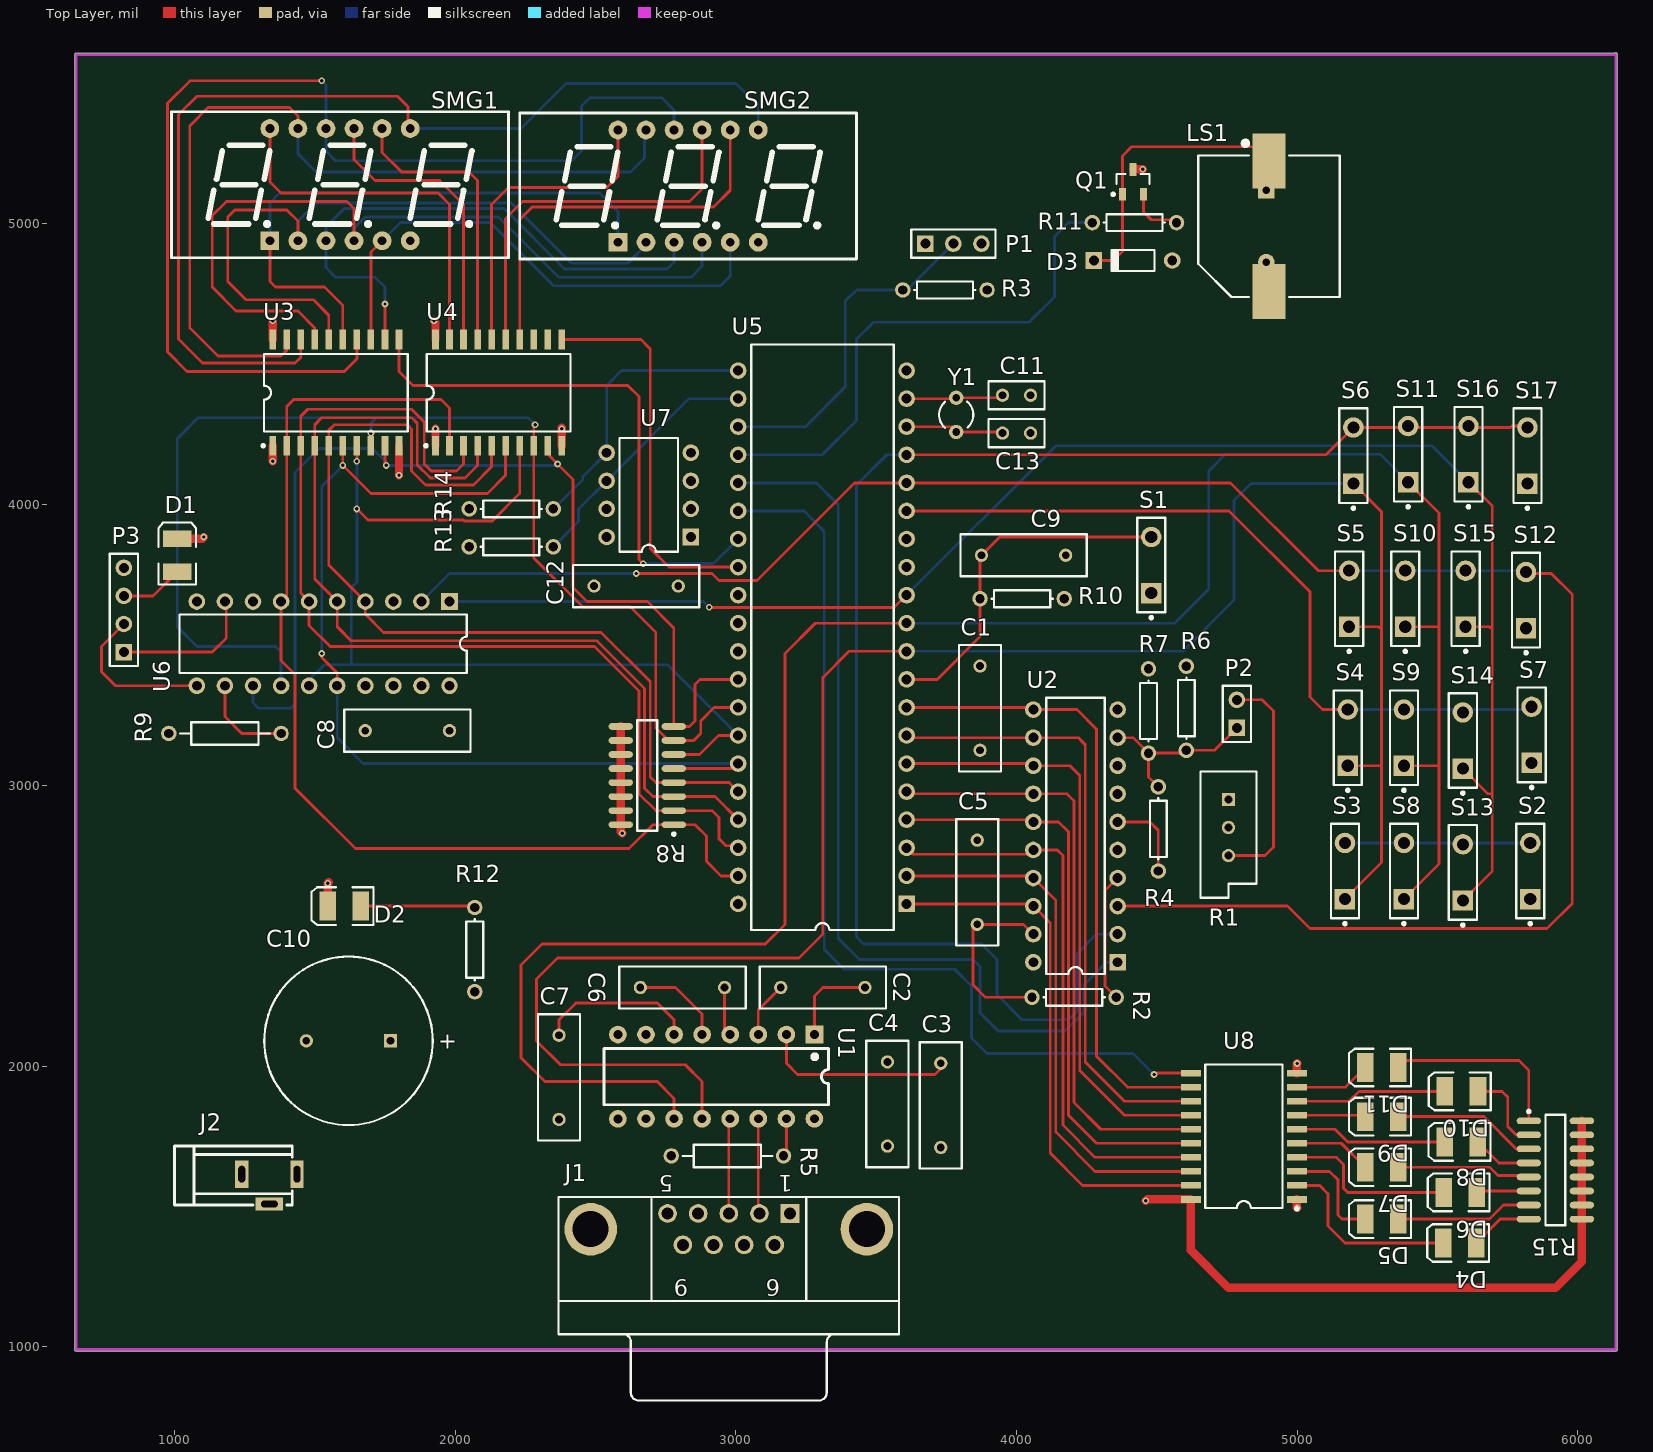
[diagram p0: Top Layer view]
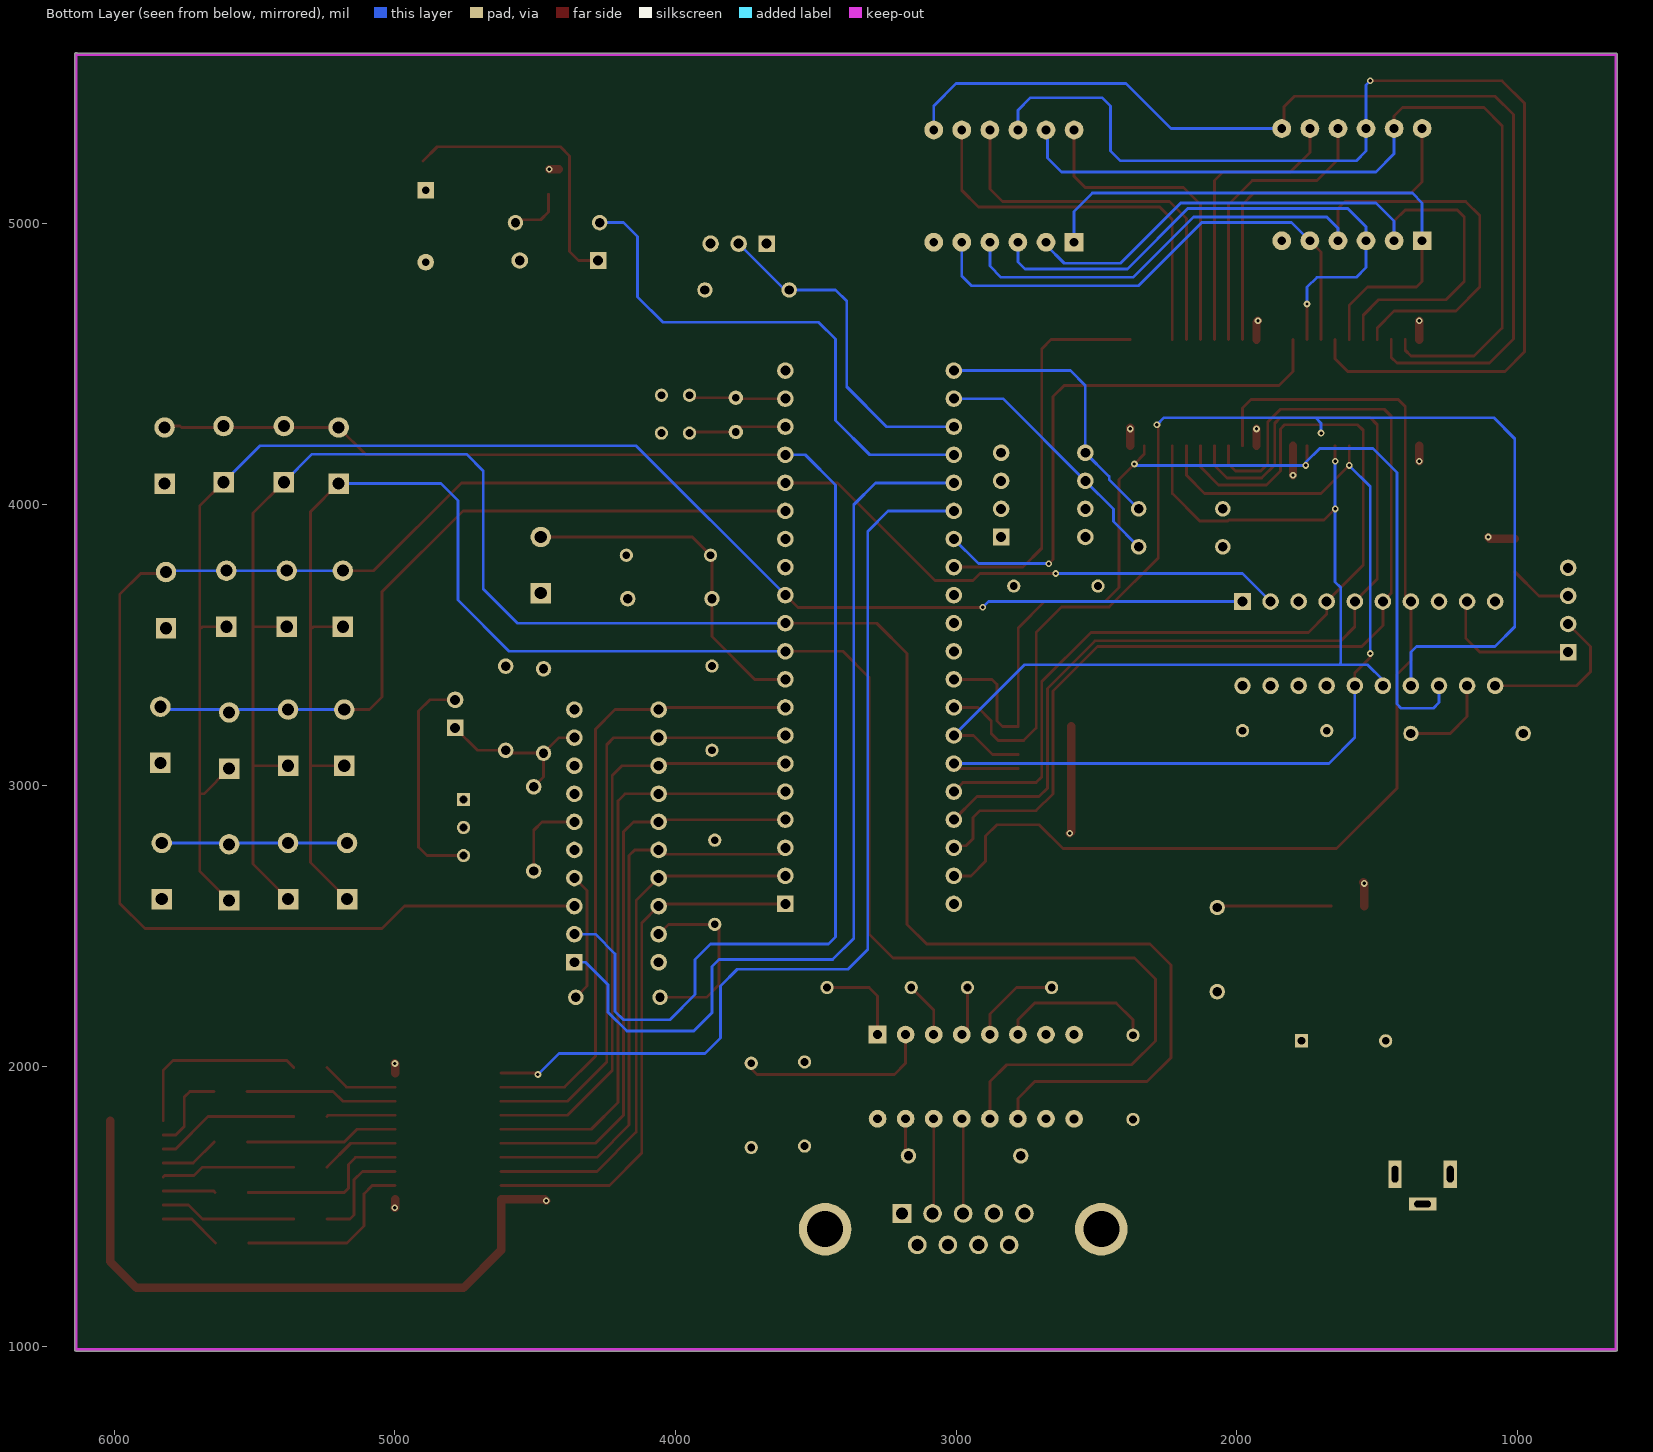
[diagram p1: Bottom Layer view, seen from below]
# Altium PCB MISC82251.PcbDoc (part 1 of 2)
Units mil, origin at the board's own origin, x right, y up, seen from the top; angles counter-clockwise.
Board outline 5495.03 x 4625.02 mil, 4 copper layers (Top Layer, VCC, GND, Bottom Layer), stack 30.634 mil thick; 74 components, 91 nets, 361 pads, 27 vias.

## Layer stack, top to bottom
Top Solder: solder mask 0.4, Solder Resist, Dk 3.5
Top Layer: signal copper 1.4
Dielectric 1: core 10, FR-4, Dk 4.2
VCC: signal copper 1.417
Dielectric 3: prepreg 5, Dk 4.2
GND: plane copper 1.417, net GND
Dielectric 2: core 10, Dk 4.2
Bottom Layer: signal copper 1.4
Bottom Solder: solder mask 0.4, Solder Resist, Dk 3.5

## Board outline
650,984.99 cw(c650,990) 644.99,990 644.99,5602.93 cw(c650,5602.93) 650,5607.94 6130,5607.94 ccw(c6130,5610) 6131.45,5608.55 cw(c6135,5605) 6140.02,5605 6140.02,990 cw(c6135,990) 6135,984.99

## Design rules (kind name [scope] priority, off if disabled: settings)
Clearance [All] p1: gap=10
HoleSize [All] p1: absolutevalues=TRUE maxlimit=10000 minlimit=1 maxpercent=80.000 minpercent=20.000
MinimumSolderMaskSliver [All] p1: minsoldermaskwidth=0
PlaneClearance [All] p1: clearance=20
PlaneConnect [All] p1: planeconnectstyle=Relief reliefexpansion=20 reliefentries=4 reliefconductorwidth=10 reliefairgap=10
PolygonConnect [All] p1: connectstyle=Relief reliefconductorwidth=10 reliefentries=4 polygonreliefangle="90 Angle" airgapwidth=10
RoutingVias [All] p1: holewidth=28 width=50 viastyle="Through Hole" minholewidth=28 minwidth=50 maxholewidth=28 maxwidth=50
SilkToSilkClearance [All] p1: silktosilkclearance=0
SilkToSolderMaskClearance [IsPad] p1: minsilkscreentomaskgap=0 clearancetoexposedcopper=TRUE
SolderMaskExpansion [All] p1: expansion=4
Width [All] p1: maxlimit=30 minlimit=10 preferedwidth=10
24 further rules are at their usual default settings.

## Components (designator, comment, footprint, x,y, rotation, side; value= is the part's Value field where it differs from the comment)
C1 "104" RAD-0.3 3870,3275 r90 top
C2 "104" RAD-0.3 3310,2280 r180 top
C3 "104" RAD-0.3 3730,1860 r90 top
C4 "104" RAD-0.3 3540,1865 r90 top
C5 "104" RAD-0.3 3860,2655 r90 top
C6 "104" RAD-0.3 2810,2280 r180 top
C7 "104" RAD-0.3 2370,1960 r90 top
C8 "104" RAD-0.3 1830,3195 r180 top
C9 "10UF" RAD-0.3 4025,3820 r0 top
C10 "100UF" RB7.6-15 1620,2090 r0 top
C11 "20PF" RAD-0.1 4000,4390 r0 top
C12 "104" RAD-0.3 2645,3710 r180 top
C13 "20PF" RAD-0.1 4000,4255 r0 top
D1 "LED3" 3.5X2.8X1.9 1010,3820 r90 top
D2 "LED3" 3.5X2.8X1.9 1605,2570 r180 top
D3 "Diode 1N4148" DO-35 4415,4870 r180 top
D4 "LED3" 3.5X2.8X1.9 5579.06,1370 r180 top
D5 "LED3" 3.5X2.8X1.9 5300.94,1455 r180 top
D6 "LED3" 3.5X2.8X1.9 5580.94,1550 r180 top
D7 "LED3" 3.5X2.8X1.9 5300.94,1640 r180 top
D8 "LED3" 3.5X2.8X1.9 5584.06,1730 r180 top
D9 "LED3" 3.5X2.8X1.9 5300.94,1820 r180 top
D10 "LED3" 3.5X2.8X1.9 5585,1910 r180 top
D11 "LED3" 3.5X2.8X1.9 5300.94,1995 r180 top
J1 "D Connector 9" DSUB1.385-2H9 2975,1045.08 r180 top
J2 "PWR2.5" DC-002 1436.85,1615 r180 top
LS1 "Buzzer" ABSM-1574 4899.45,5224.33 r270 top
P1 "DS18B20" HDR1X3 3675,4930 r0 top
P2 "Header 2" HDR1X2 4785,3205 r90 top
P3 "Header 4" HDR1X4 820,3475 r90 top
Q1 "PNP" SOT-23B_N 4415,5150 r90 top
R1 "RPot" VR5 4755,2850 r270 top
R2 "10K" AXIAL-0.3 4205,2245 r0 top
R3 "4.7K" AXIAL-0.3 3745,4765 r0 top
R4 "10K" AXIAL-0.3 4505,2845 r270 top
R5 "0" AXIAL-0.4 2970,1680 r0 top
R6 "1k" AXIAL-0.3 4605,3275 r270 top
R7 "1K" AXIAL-0.3 4470,3265 r90 top
R8 "Res Pack3" SO-16_N 2684.49,3035 r180 top
R9 "0" AXIAL-0.4 1180,3185 r180 top
R10 "10K" AXIAL-0.3 4020,3665 r180 top
R11 "2K" AXIAL-0.3 4420,5005 r180 top
R12 "2K" AXIAL-0.3 2070,2415 r270 top
R13 "4.7K" AXIAL-0.3 2200,3850 r180 top
R14 "4.7K" AXIAL-0.3 2200,3985 r180 top
R15 "Res Pack3" SO-16_N 5919.49,1630 r0 top
S1 "SW-PB" SPST-2 4480,3785 r90 top
S2 "SW-PB" SPST-2 5830,2695 r90 top
S3 "SW-PB" SPST-2 5170,2695 r90 top
S4 "SW-PB" SPST-2 5180,3170 r90 top
S5 "SW-PB" SPST-2 5185,3665 r90 top
S6 "SW-PB" SPST-2 5200,4175 r90 top
S7 "SW-PB" SPST-2 5835,3180 r90 top
S8 "SW-PB" SPST-2 5380,2695 r90 top
S9 "SW-PB" SPST-2 5380,3170 r90 top
S10 "SW-PB" SPST-2 5385,3665 r90 top
S11 "SW-PB" SPST-2 5395,4180 r90 top
S12 "SW-PB" SPST-2 5815,3660 r90 top
S13 "SW-PB" SPST-2 5590,2690 r90 top
S14 "SW-PB" SPST-2 5590,3160 r90 top
S15 "SW-PB" SPST-2 5600,3665 r90 top
S16 "SW-PB" SPST-2 5610,4180 r90 top
S17 "SW-PB" SPST-2 5820,4175 r90 top
SMG1 "3931A" "SMG 0.39-3P" 1590,5140 r0 top
SMG2 "3931A" "SMG 0.39-3P" 2830,5135 r0 top
U1 "MAX232ESE" DIP16 3280,2112.5 r270 top
U2 "ADC0804CN" N020 4210,2820 r90 top
U3 "MC74HC573DW" 751D-03 1575,4398.98 r0 top
U4 "MC74HC573DW" 751D-03 2155,4398.98 r0 top
U5 "P89C51RC2HBP" SOT129-1 3308.53,3527.76 r90 top
U6 "DAC0832LCJ" J20A 1530,3505 r180 top
U7 "M24C02BN6" PSDIP8A 2690,4035 r90 top
U8 "MC74HC573ADW" 751D-05 4810,1750 r90 top
Y1 "XTAL" R38 3785,4320 r180 top

## Footprints (in the part's own frame and the unit in brackets; to place one, negate y for a bottom-side part, rotate by r counter-clockwise, add the part's x,y. Pads: shape width x height; smd on the part's side, far side on the other; paste and mask are expansions set on the pad)
3.5X2.8X1.9 [mm] "SM LED; 2 C-Bend Leads; Body 3.5 x 2.8 x 1.9 mm, inc leads (LxWxH typ)"
  rect 1.5x2.6 smd: 1(-1.5,0) 2(1.5,0)
  silkscreen extent -2.65,-1.7 2.95,1.7
751D-03 [mm] "Small Outline; 20 Leads; Body Width 7.5 mm; Pitch 1.27 mm"
  rect 0.6x1.8 smd: 1(-5.715,-4.8) 2(-4.445,-4.8) 3(-3.175,-4.8) 4(-1.905,-4.8) 5(-0.635,-4.8) 6(0.635,-4.8) 7(1.905,-4.8) 8(3.175,-4.8) 9(4.445,-4.8) 10(5.715,-4.8) 11(5.715,4.8) 12(4.445,4.8) 13(3.175,4.8) 14(1.905,4.8) 15(0.635,4.8) 16(-0.635,4.8) 17(-1.905,4.8) 18(-3.175,4.8) 19(-4.445,4.8) 20(-5.715,4.8)
  silkscreen extent -6.7,-4.92 6.5,3.5
751D-05 [mm] "Small Outline; 20 Leads; Body Width 7.5 mm; Pitch 1.27 mm"
  rect 0.6x1.8 smd: 1(-5.715,-4.8) 2(-4.445,-4.8) 3(-3.175,-4.8) 4(-1.905,-4.8) 5(-0.635,-4.8) 6(0.635,-4.8) 7(1.905,-4.8) 8(3.175,-4.8) 9(4.445,-4.8) 10(5.715,-4.8) 11(5.715,4.8) 12(4.445,4.8) 13(3.175,4.8) 14(1.905,4.8) 15(0.635,4.8) 16(-0.635,4.8) 17(-1.905,4.8) 18(-3.175,4.8) 19(-4.445,4.8) 20(-5.715,4.8)
  silkscreen extent -6.7,-4.93 6.5,3.5
ABSM-1574 [mm] "Magnetic Transducer Buzzer"
  rect 5x3 smd: 1(0,0) 2(11.8,0)
  rect 1.5x1.5 hole 0.7: 1A(2.65,-0.24)
  round 1.5 hole 0.7: 2A(9.15,-0.24)
  silkscreen extent -1.83,-6.4 12.3,6.4
AXIAL-0.3 [mm] "Axial Device, Thru-Hole; 2 Leads; 0.3 in Pin Spacing"
  round 1.4 hole 0.85: 1(-3.81,0) 2(3.81,0)
  silkscreen extent -2.77,-0.76 2.77,0.76
AXIAL-0.4 [mm] "Axial Device, Thru-Hole; 2 Leads; 0.4 in Pin Spacing"
  round 1.4 hole 0.85: 1(-5.08,0) 2(5.08,0)
  silkscreen extent -4.06,-1.02 4.06,1.02
DC-002 [mm] "3.5X1.1mm"
  rect 1.2x2.5 hole 0.6 slot 1.5 at 90 deg: 1(0,0) 2(5,0)
  rect 2.5x1.2 hole 0.6 slot 1.5 at 0 deg: 3(2.5,2.7)
  silkscreen extent 0.43,-2.54 11.1,2.79, body extent -0.25,-2.55 11.05,2.8, height 7.3
DIP16 [mm]
  rect 1.6x1.6 hole 0.813: 1(0,0)
  round 1.6 hole 0.813: 2(0,-2.54) 3(0,-5.08) 4(0,-7.62) 5(0,-10.16) 6(0,-12.7) 7(0,-15.24) 8(0,-17.78) 9(7.627,-17.78) 10(7.62,-15.24) 11(7.62,-12.7) 12(7.62,-10.16) 13(7.62,-7.62) 14(7.62,-5.08) 15(7.62,-2.54) 16(7.62,0)
  silkscreen extent 1.27,-19.05 6.35,1.27, body extent -0.12,-18.76 7.75,1.24, height 5.1
DO-35 [mm] "Diode, Axial; Body 3.8 x 1.9 mm (LxDia. max), Lead Dia. 0.53 mm (max)"
  round 1.5 hole 0.9: 1(-3.55,0)
  rect 1.5x1.5 hole 0.9: 2(3.55,0)
  silkscreen extent -1.95,-0.95 2.05,0.95
DSUB1.385-2H9 [mm] "Connector; D Subminiature; 9 Position; Right Angle; Pitch 1.385 mm"
  rect 1.69x1.69 hole 1.09: 1(-5.54,-10.92)
  round 1.69 hole 1.09: 2(-2.77,-10.92) 3(0,-10.92) 4(2.77,-10.92) 5(5.54,-10.92) 6(-4.155,-8.08) 7(-1.385,-8.08) 8(1.385,-8.08) 9(4.155,-8.08)
  round 4.76 hole 3.26: 10(-12.495,-9.5) 11(12.495,-9.5)
  silkscreen extent -15.4,-12.4 15.4,6
HDR1X2 [mm] "Connector; Header; 2 Position"
  rect 1.5x1.5 hole 0.9: 1(0,0)
  round 1.5 hole 0.9: 2(2.54,0)
  silkscreen extent -1.27,-1.27 3.81,1.27
HDR1X3 [mm] "Connector; Header; 3 Position"
  rect 1.5x1.5 hole 0.9: 1(0,0)
  round 1.5 hole 0.9: 2(2.54,0) 3(5.08,0)
  silkscreen extent -1.27,-1.27 6.35,1.27
HDR1X4 [mm] "Connector; Header; 4 Position"
  rect 1.5x1.5 hole 0.9: 1(0,0)
  round 1.5 hole 0.9: 2(2.54,0) 3(5.08,0) 4(7.62,0)
  silkscreen extent -1.27,-1.27 8.89,1.27
J20A [mm] "DIP; 20 Leads; Row Spacing 7.62 mm; Pitch 2.54 mm"
  rect 1.5x1.5 hole 0.9: 1(-11.43,-3.81)
  round 1.5 hole 0.9: 2(-8.89,-3.81) 3(-6.35,-3.81) 4(-3.81,-3.81) 5(-1.27,-3.81) 6(1.27,-3.81) 7(3.81,-3.81) 8(6.35,-3.81) 9(8.89,-3.81) 10(11.43,-3.81) 11(11.43,3.81) 12(8.89,3.81) 13(6.35,3.81) 14(3.81,3.81) 15(1.27,3.81) 16(-1.27,3.81) 17(-3.81,3.81) 18(-6.35,3.81) 19(-8.89,3.81) 20(-11.43,3.81)
  silkscreen extent -13,-2.65 13,2.65
N020 [mm] "DIP; 20 Leads; Row Spacing 7.62 mm; Pitch 2.54 mm"
  rect 1.5x1.5 hole 0.9: 1(-11.43,-3.81)
  round 1.5 hole 0.9: 2(-8.89,-3.81) 3(-6.35,-3.81) 4(-3.81,-3.81) 5(-1.27,-3.81) 6(1.27,-3.81) 7(3.81,-3.81) 8(6.35,-3.81) 9(8.89,-3.81) 10(11.43,-3.81) 11(11.43,3.81) 12(8.89,3.81) 13(6.35,3.81) 14(3.81,3.81) 15(1.27,3.81) 16(-1.27,3.81) 17(-3.81,3.81) 18(-6.35,3.81) 19(-8.89,3.81) 20(-11.43,3.81)
  silkscreen extent -12.5,-2.65 12.5,2.65
PSDIP8A [mm] "DIP; 8 Leads; Row Spacing 7.62 mm; Pitch 2.54 mm"
  rect 1.5x1.5 hole 0.9: 1(-3.81,-3.81)
  round 1.5 hole 0.9: 2(-1.27,-3.81) 3(1.27,-3.81) 4(3.81,-3.81) 5(3.81,3.81) 6(1.27,3.81) 7(-1.27,3.81) 8(-3.81,3.81)
  silkscreen extent -5.15,-2.65 5.15,2.65
R38 [mm] "Crystal, Thru-Hole; 2 Leads; Body 3.1 x 8.2 mm (Dia.xH)"
  round 1.3 hole 0.7: 1(0,1.55) 2(0,-1.55)
  silkscreen extent -1.55,-1.19 1.55,1.17
RAD-0.1 [mm] "Radial Cap, Thru-Hole; 2 Leads; 0.1 in Pin Spacing"
  round 1.2 hole 0.7: 1(-1.27,0) 2(1.27,0)
  silkscreen extent -2.54,-1.27 2.54,1.27
RAD-0.3 [mm] "Radial Cap, Thru-Hole; 2 Leads; 0.3 in Pin Spacing"
  round 1.2 hole 0.7: 1(-3.81,0) 2(3.81,0)
  silkscreen extent -5.71,-1.91 5.71,1.91
RB7.6-15 [mm] "Polarized Capacitor (Radial); 2 Leads"
  rect 1.2x1.2 hole 0.7: 1(3.81,0)
  round 1.2 hole 0.7: 2(-3.81,0)
  silkscreen extent -7.62,-7.62 7.62,7.62
"SMG 0.39-3P" [mm] "30.2*13*7mm(长宽厚)"
  rect 1.7x1.7 hole 0.8: 1(-6.35,-5.08)
  round 1.7 hole 0.8: 2(-3.81,-5.08) 3(-1.27,-5.08) 4(1.27,-5.08) 5(3.81,-5.08) 6(6.35,-5.08) 7(6.35,5.08) 8(3.81,5.08) 9(1.27,5.08) 10(-1.27,5.08) 11(-3.81,5.08) 12(-6.35,5.08)
  silkscreen extent -15.24,-6.6 15.24,6.6, body extent -15.01,-6.5 15.01,6.5, height 7
SO-16_N [mm] "SOIC, 16-Leads, Body 9.9x3.9mm, Pitch 1.27mm, IPC Medium Density"
  oval 2.2x0.6 smd: 1(-2.4,4.445) 2(-2.4,3.175) 3(-2.4,1.905) 4(-2.4,0.635) 5(-2.4,-0.635) 6(-2.4,-1.905) 7(-2.4,-3.175) 8(-2.4,-4.445) 9(2.4,-4.445) 10(2.4,-3.175) 11(2.4,-1.905) 12(2.4,-0.635) 13(2.4,0.635) 14(2.4,1.905) 15(2.4,3.175) 16(2.4,4.445)
  silkscreen extent -2.53,-5 0.9,5.42, body extent -2,-5 2,5, height 1.75
SOT129-1 [mm] "DIP; 40 Leads; Row Spacing 15.24 mm; Pitch 2.54 mm"
  rect 1.5x1.5 hole 0.9: 1(-24.13,-7.62)
  round 1.5 hole 0.9: 2(-21.59,-7.62) 3(-19.05,-7.62) 4(-16.51,-7.62) 5(-13.97,-7.62) 6(-11.43,-7.62) 7(-8.89,-7.62) 8(-6.35,-7.62) 9(-3.81,-7.62) 10(-1.27,-7.62) 11(1.27,-7.62) 12(3.81,-7.62) 13(6.35,-7.62) 14(8.89,-7.62) 15(11.43,-7.62) 16(13.97,-7.62) 17(16.51,-7.62) 18(19.05,-7.62) 19(21.59,-7.62) 20(24.13,-7.62) 21(24.13,7.62) 22(21.59,7.62) 23(19.05,7.62) 24(16.51,7.62) 25(13.97,7.62) 26(11.43,7.62) 27(8.89,7.62) 28(6.35,7.62) 29(3.81,7.62) 30(1.27,7.62) 31(-1.27,7.62) 32(-3.81,7.62) 33(-6.35,7.62) 34(-8.89,7.62) 35(-11.43,7.62) 36(-13.97,7.62) 37(-16.51,7.62) 38(-19.05,7.62) 39(-21.59,7.62) 40(-24.13,7.62)
  silkscreen extent -26.5,-6.45 26.5,6.45
SOT-23B_N [mm] "SOT23, 3-Leads, Body 2.9x1.3mm, Pitch 0.95mm, Lead Span 2.4mm, IPC Medium Density"
  rect 1.15x0.6 smd: 1(-1.125,0.95) 2(-1.125,-0.95) 3(1.125,0)
  silkscreen extent -1.25,-1.5 0.7,1.92, body extent -0.7,-1.5 0.7,1.5, height 1.14
SPST-2 [mm] "Switch; 2 Leads"
  rect 1.85x1.85 hole 1.1: 1(-2.54,0)
  round 1.85 hole 1.1: 2(2.54,0)
  silkscreen extent -4.89,-1.27 4.28,1.27
VR5 [mm] "Thru-Hole; 3 Leads"
  rect 1.2x1.2 hole 0.7: 1(-2.54,0)
  round 1.2 hole 0.7: 2(0,0) 3(2.54,0)
  silkscreen extent -5.08,-2.54 6.35,2.54

## Part data
C1 C2 C3 C4 C5 C6 C7 C8 C9 C11 C12 C13: library part Cap, "Capacitor"
C10: library part "Cap Pol1", "Polarized Capacitor (Radial)"
D1 D2 D4 D5 D6 D7 D8 D9 D10 D11: "Typical BLUE SiC LED"
D3: "High Conductance Fast Diode"
J1: "Receptacle Assembly, 9 Position, Right Angle"
J2: library part DC_Socket
LS1: "Magnetic Transducer Buzzer"
P1: library part "Header 3", "Header, 3-Pin"
P2: "Header, 2-Pin"
P3: "Header, 4-Pin"
Q1: "PNP Bipolar Transistor"
R1: "Potentiometer"
R2 R3 R4 R6 R7 R10 R11 R12 R13 R14: library part Res1, "Resistor"
R5 R9: library part Res2, "Resistor"
R8 R15: "Isolated Resistor Network"
S1 S2 S3 S4 S5 S6 S7 S8 S9 S10 S11 S12 S13 S14 S15 S16 S17: "Switch"
SMG1 SMG2: "0.39 inch 3-digit common-cathode LED display"
U1: "+5V Powered, Multi-Channel RS-232 Driver/Receiver"
U2: "8-Bit Analog-to-Digital Converter with Differential Inputs"
U3 U4 U8: "Octal 3-State Non-Inverting Transparent Latch"
U5: "80C51 8-Bit Flash Microcontroller Family, 32 kB ISP/IAP Flash with 512 B RAM."
U6: "8-Bit uP-Compatible, Double-Buffered Digital-to-Analog Converter"
U7: "2Kbit Serial IIC Bus EEPROM"
Y1: "Crystal Oscillator"

## Via types
v1: diameter 24, hole 12, Top Layer to Bottom Layer, 27 vias

## Nets (pads, with @x,y where several pads share a name; then routed paths per layer and width w, separated by ;. In a path a pad name is that pad's centre, name@x,y a point inside that pad or via, vN(x,y) a via of type N, cw(c..) or ccw(c..) an arc to the next point about the centre after c; other vN are vias at no path point)
18B20: P1.2 R3.1 U5.23 | length 1215.3
  Bottom Layer w10: U5.23 3247.76,4277.76 3390,4420 3390,4725 3430,4765 R3.1 3610,4765 P1.2
A: SMG1.11 SMG2.11 U3.19 | length 3096.7
  Top Layer w10: U3.19 1400,4550 1380,4530 1155,4530 1055,4630 1055,5350 1120,5415 1410,5415 1440,5385 SMG1.11
  Bottom Layer w10: SMG1.11 1440,5250 1505,5185 2625,5185 2675,5235 2675,5330 SMG2.11
ALE: U5.30
B: SMG1.7 SMG2.7 U3.18 | length 3706.4
  Top Layer w10: U3.18 1450,4525 1430,4505 1100,4505 1015,4590 1015,5390 1080,5455 1795,5455 1832.5,5417.5 1832.5,5347.5 SMG1.7
  Bottom Layer w10: SMG1.7 2235,5340 2395,5500 3000,5500 3080,5420 SMG2.7
C: SMG1.4 SMG2.4 U3.17 | length 2865.4
  Top Layer w10: U3.17 1500,4630 1440,4690 1220,4690 1135,4775 1135,5030 1185,5080 1615,5080 1640,5055 SMG1.4
  Bottom Layer w10: SMG1.4 1640,4985 1680,5025 2155,5025 2370,4810 2840,4810 2880,4850 SMG2.4
CSAD: U2.1 U5.25 | length 3321.1
  Bottom Layer w10: U5.25 3287.24,4077.76 3365,4000 3365,2455 3440,2380 3845,2380 3870,2355 3870,2190 3935,2125 4173.28,2125 4240,2191.72 4240,2290 4320,2370 U2.1
D: SMG1.2 SMG2.2 U3.16 | length 2536.6
  Top Layer w10: SMG1.2 1440,5010 1400,5050 1215,5050 1190,5025 1190,4795 1255,4730 1495,4730 1550,4675 U3.16
  Bottom Layer w10: SMG1.2 1440,5010 1505,5075 2200,5075 2415,4860 2615,4860 2680,4925 SMG2.2